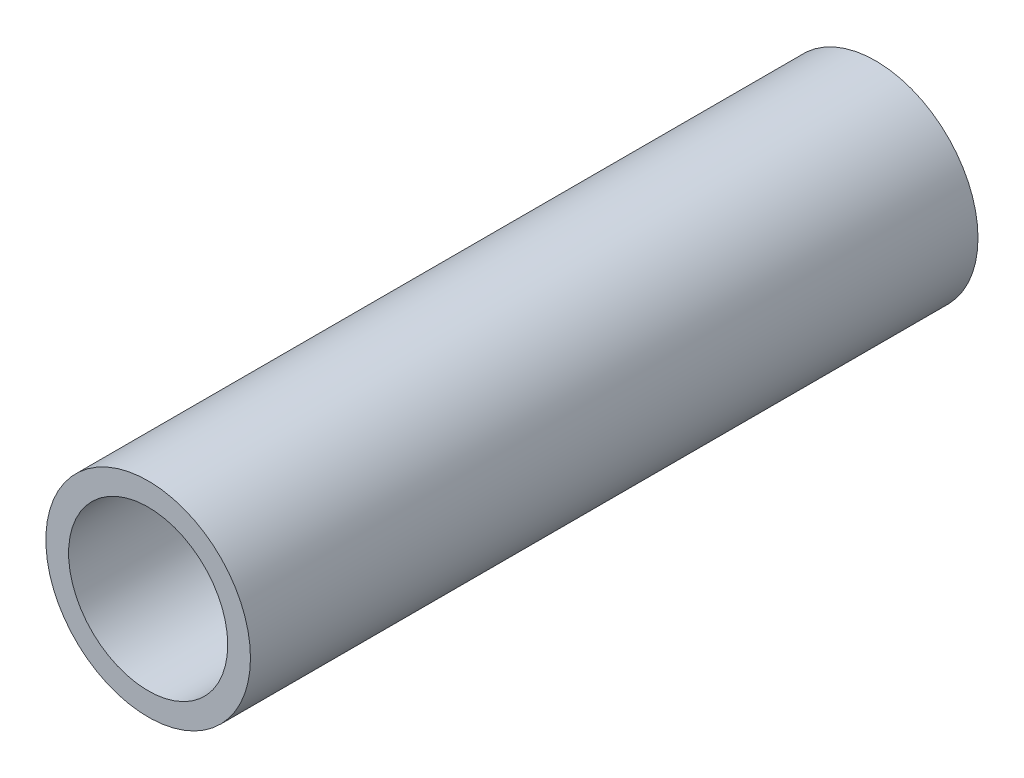
from build123d import *

# Parameters (mm, degrees)
SKETCH1_R           = 4.5
SKETCH1_R_2         = 3.5
BOSS_EXTRUDE1_DEPTH = 32


with BuildPart() as part:
    # Sketch1 → Boss-Extrude1 (new body)
    with BuildSketch(Plane.XY):
        Circle(SKETCH1_R)
        Circle(SKETCH1_R_2, mode=Mode.SUBTRACT)
    extrude(amount=BOSS_EXTRUDE1_DEPTH)


solid = part.part
